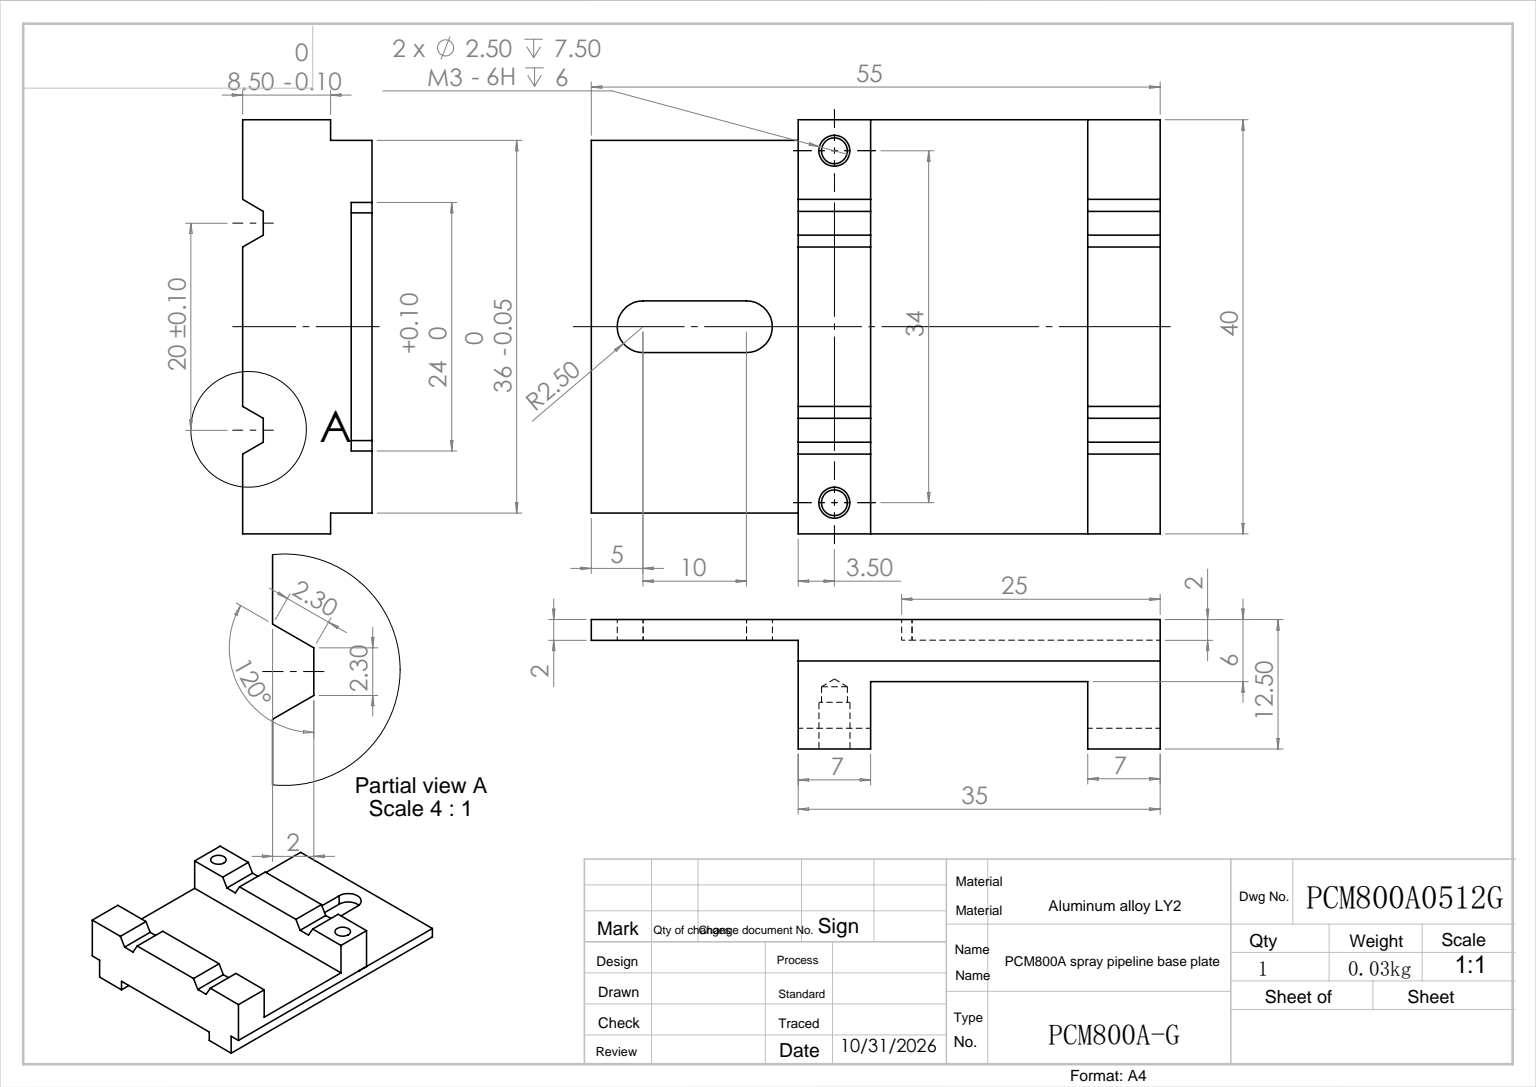
SolidWorks part; units mm, degrees
ref_plane "前视基准面" through (0, 0, 0) normal (0, 0, 1) x (1, 0, 0)
ref_plane "上视基准面" through (0, 0, 0) normal (0, 1, 0) x (1, 0, 0)
ref_plane "右视基准面" through (0, 0, 0) normal (1, 0, 0) x (0, 0, -1)
sketch "草图1" plane through (0, 0, 0) normal (0, 0, 1) x (1, 0, 0)
  line L1 (0, 0) -> (35, 0)
  line L2 (0, 0) -> (0, 4)
  line L3 (0, 4) -> (35, 4)
  line L4 (35, 0) -> (35, 4)
  dimension "D1" = 4
  dimension "D2" = 35
extrude "拉伸1" add sketch "草图1" along normal blind 40
sketch "草图2" plane through (0, 4, 0) normal (0, 1, 0) x (-1, 0, 0)
  line L0 (-35, 0) -> (0, 0) construction
  line L1 (0, 40) -> (-7, 40)
  line L2 (0, 40) -> (0, 0)
  line L3 (0, 0) -> (-7, 0)
  line L4 (-7, 40) -> (-7, 0)
  dimension "D1" = 7
extrude "拉伸2" add sketch "草图2" against normal blind 12
hole_wizard "M3 螺纹孔1" positions "草图7" profile "草图6" tap size "M3" standard "GB"
sketch "草图7" plane through (0, -8, 0) normal (0, -1, 0) x (1, 0, 0)
  line L0 (0, 20) -> (35, 20) construction
  line L3 (7, 0) -> (0, 0) construction
  line L4 (35, 40) -> (35, 0) construction
  point P0 (3.5, 3)
  point P9 (3.5, 37)
  dimension "D1" = 3.5
  dimension "D2" = 3
sketch "草图6" plane through (3.5, -8, 3) normal (1, 0, 0) x (0, 0, -1)
  line L0 (0, 0) -> (0, 8.2511)
  line L1 (0, 8.2511) -> (1.25, 7.5)
  line L2 (1.25, 7.5) -> (1.25, 6)
  line L3 (1.25, 6) -> (1.5, 6)
  line L4 (1.5, 6) -> (1.5, 0)
  line L5 (1.5, 0) -> (0, 0)
  line L10 (0, 8.2511) -> (-1.25, 7.5) construction
  line L11 (0, -6.35) -> (0, 107.95) construction
  dimension "蹟恇謂郰芛眻噤" = 2.5
  dimension "蹟恇謂郰芛旮僅" = 7.5
  dimension "蹟恇翋眻噤" = 3
  dimension "蹟恇旮僅" = 6
  dimension "絳芛褒僅" = 118
sketch "草图9" plane through (0, 0, 0) normal (0, -1, 0) x (1, 0, 0)
  line L0 (35, 40) -> (35, 0) construction
  line L1 (35, 40) -> (28, 40)
  line L2 (35, 40) -> (35, 0)
  line L3 (35, 0) -> (28, 0)
  line L4 (28, 40) -> (28, 0)
  line L5 (7, 40) -> (35, 40) construction
  line L6 (7, 0) -> (35, 0) construction
  dimension "D1" = 7
extrude "拉伸3" add sketch "草图9" along normal blind 10
sketch "草图14" plane through (35, 0, 0) normal (1, 0, 0) x (0, 0, -1)
  line L0 (-40, -10) -> (-40, 4) construction
  line L1 (0, -10) -> (-40, -10)
  line L2 (0, -10) -> (0, -6.5)
  line L3 (0, -6.5) -> (-40, -6.5)
  line L4 (-40, -10) -> (-40, -6.5)
  dimension "D1" = 3.5
extrude "切除-拉伸5" cut sketch "草图14" against normal through all
sketch "草图15" plane through (0, 0, 0) normal (-1, 0, 0) x (0, 0, 1)
  line L1 (0, 4) -> (2, 4)
  line L2 (0, 4) -> (0, 2)
  line L3 (0, 2) -> (2, 2)
  line L4 (2, 4) -> (2, 2)
  line L5 (40, 4) -> (38, 4)
  line L6 (40, 4) -> (40, 2)
  line L7 (40, 2) -> (38, 2)
  line L8 (38, 4) -> (38, 2)
  dimension "D1" = 2
  dimension "D2" = 2
  dimension "D3" = 2
  dimension "D4" = 2
extrude "切除-拉伸6" cut sketch "草图15" against normal through all
sketch "草图17" plane through (0, 4, 0) normal (0, 1, 0) x (1, 0, 0)
  line L0 (0, -38) -> (0, -2) construction
  line L1 (-20, -2) -> (35, -2)
  line L2 (-20, -2) -> (-20, -38)
  line L4 (10, -8) -> (10, -32)
  line L5 (35, -38) -> (35, -2) construction
  line L7 (35, -38) -> (-20, -38)
  line L8 (35, -38) -> (35, -32)
  line L9 (35, -32) -> (10, -32)
  line L12 (35, -2) -> (35, -8)
  line L13 (35, -8) -> (10, -8)
  dimension "D1" = 20
  dimension "D2" = 25
  dimension "D3" = 6
  dimension "D4" = 6
extrude "拉伸5" add sketch "草图17" along normal blind 2
sketch "草图18" plane through (0, 0, 0) normal (-1, 0, 0) x (0, 0, 1)
  line L6 (31.15, -4.5081) -> (28.85, -4.5081)
  line L7 (28.85, -4.5081) -> (27.7, -6.5)
  line L8 (27.7, -6.5) -> (28.85, -8.4919)
  line L9 (28.85, -8.4919) -> (31.15, -8.4919)
  line L10 (31.15, -8.4919) -> (32.3, -6.5)
  line L11 (32.3, -6.5) -> (31.15, -4.5081)
  line L12 (31.15, -4.5081) -> (28.85, -4.5081)
  line L13 (28.85, -4.5081) -> (27.7, -6.5)
  line L14 (27.7, -6.5) -> (28.85, -8.4919)
  line L15 (28.85, -8.4919) -> (31.15, -8.4919)
  line L16 (31.15, -8.4919) -> (32.3, -6.5)
  line L17 (32.3, -6.5) -> (31.15, -4.5081)
  dimension "D1" = 0
extrude "切除-拉伸7" cut sketch "草图18" against normal through all
ref_plane "基准面1" through (0, 0, 20) normal (0, 0, -1) x (-1, 0, 0)
mirror "镜向1" about plane through (0, 0, 20) normal (0, 0, -1) of "切除-拉伸7"
sketch "草图19" plane through (35, 0, 0) normal (1, 0, 0) x (0, 0, -1)
  line L0 (-28.85, -4.5081) -> (-27.7, -6.5) construction
  line L1 (-31.15, -4.5081) -> (-28.85, -4.5081) construction
  line L2 (-32.3, -6.5) -> (-31.15, -4.5081) construction
  line L3 (-28.85, -4.5081) -> (-27.7, -6.5)
  line L4 (-31.15, -4.5081) -> (-28.85, -4.5081)
  line L5 (-32.3, -6.5) -> (-31.15, -4.5081)
  line L6 (-32.3, -6.5) -> (-27.7, -6.5)
fillet "圆角1" radius 1 2 edges at (10, 5, 32) (10, 5, 8)
sketch "草图20" plane through (0, 4, 0) normal (0, -1, 0) x (1, 0, 0)
  line L0 (-15, 20) -> (-5, 20) construction
  line L1 (-15, 22.5) -> (-5, 22.5)
  line L2 (-15, 17.5) -> (-5, 17.5)
  line L3 (0, 2) -> (-20, 2) construction
  line L4 (-20, 2) -> (-20, 38) construction
  arc A0 (-15, 22.5) -> (-15, 17.5) centre (-15, 20) ccw
  arc A1 (-5, 17.5) -> (-5, 22.5) centre (-5, 20) ccw
  point P2 (-10, 20)
  dimension "D1" = 18
  dimension "D2" = 2.5
  dimension "D3" = 5
  dimension "D4" = 10
extrude "切除-拉伸8" cut sketch "草图20" against normal through all
